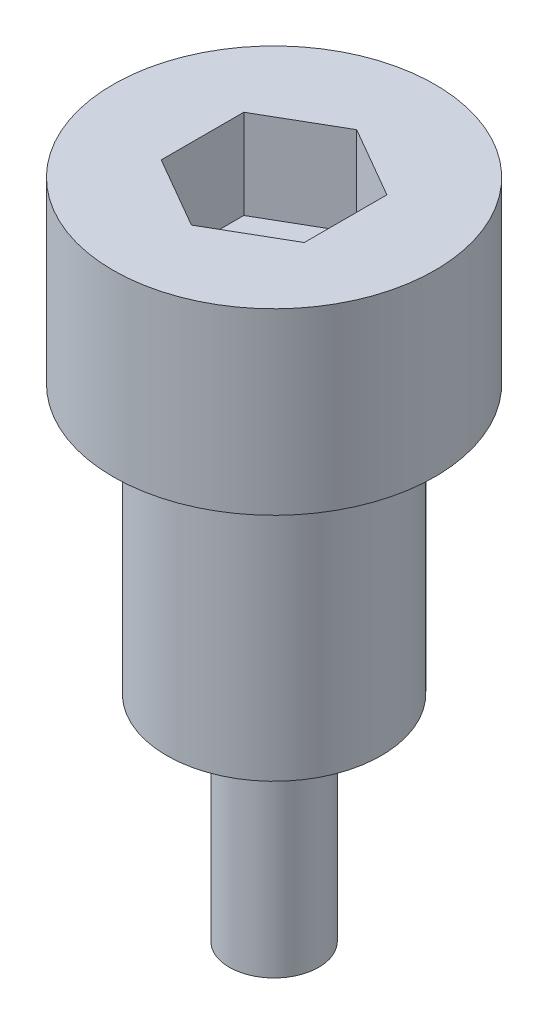
SolidWorks part; units mm, degrees
material "42CrMo"
ref_plane "Front Plane" through (0, 0, 0) normal (0, 0, 1) x (1, 0, 0)
ref_plane "Top Plane" through (0, 0, 0) normal (0, 1, 0) x (1, 0, 0)
ref_plane "Right Plane" through (0, 0, 0) normal (1, 0, 0) x (0, 0, -1)
sketch "Sketch1" plane through (0, 0, 0) normal (0, 1, 0) x (1, 0, 0)
  circle A0 centre (0, 0) radius 2.5
  dimension "D1" = 5
extrude "Boss-Extrude1" add sketch "Sketch1" along normal blind 12
cosmetic thread "Cosmetic Thread1" parameters "D2"=4.134
sketch "Sketch2" plane through (0, 12, 0) normal (0, 1, 0) x (1, 0, 0)
  circle A0 centre (0, 0) radius 6
  dimension "D1" = 12
extrude "Boss-Extrude2" add sketch "Sketch2" along normal blind 15
sketch "Sketch3" plane through (0, 27, 0) normal (0, 1, 0) x (1, 0, 0)
  circle A0 centre (0, 0) radius 9
  dimension "D1" = 18
extrude "Boss-Extrude3" add sketch "Sketch3" along normal blind 10
sketch "Sketch4" plane through (0, 37, 0) normal (0, 1, 0) x (1, 0, 0)
  line L1 (0, 4.6188) -> (-4, 2.3094)
  line L2 (-4, 2.3094) -> (-4, -2.3094)
  line L3 (-4, -2.3094) -> (0, -4.6188)
  line L4 (0, -4.6188) -> (4, -2.3094)
  line L5 (4, -2.3094) -> (4, 2.3094)
  line L6 (4, 2.3094) -> (0, 4.6188)
  circle A0 centre (0, 0) radius 4 construction
  dimension "D2" = 8
extrude "Cut-Extrude1" cut sketch "Sketch4" against normal blind 5
